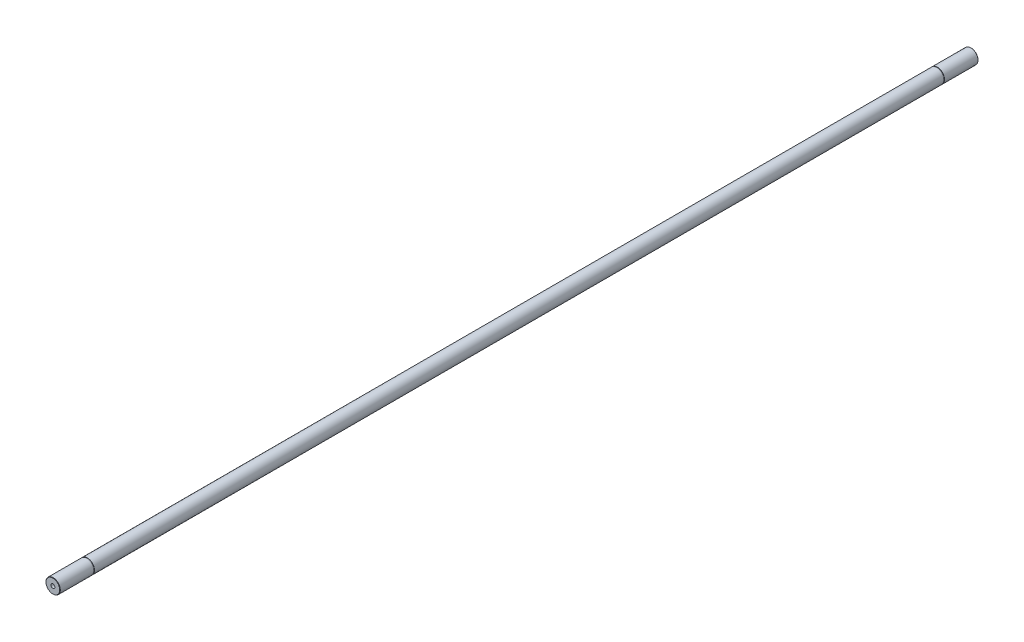
SolidWorks part; units mm, degrees
ref_plane "前视基准面" through (0, 0, 0) normal (0, 0, 1) x (1, 0, 0)
ref_plane "上视基准面" through (0, 0, 0) normal (0, 1, 0) x (1, 0, 0)
ref_plane "右视基准面" through (0, 0, 0) normal (1, 0, 0) x (0, 0, -1)
sketch "草图1" plane through (0, 0, 0) normal (0, 0, 1) x (1, 0, 0)
  circle A0 centre (0, 0) radius 12.5
  dimension "D1" = 25
extrude "凸台-拉伸1" add sketch "草图1" along normal blind 1600
chamfer "倒角1" distance 0.5 angle 45 2 edges at (12.5, 0, 0) (12.5, 0, 1600)
sketch "草图2" plane through (0, 0, 0) normal (0, 1, 0) x (1, 0, 0)
  line L0 (12.5, -1599.5) -> (12.5, -0.5) construction
  line L1 (12.5, -1539.9) -> (11.95, -1539.9)
  line L2 (12.5, -1539.9) -> (12.5, -1541.2)
  line L3 (12.5, -1541.2) -> (11.95, -1541.2)
  line L4 (11.95, -1539.9) -> (11.95, -1541.2)
  line L6 (0, -1599.5) -> (0, -1417.9402) construction
  line L7 (12.5, -1599.5) -> (-12.5, -1599.5) construction
  line L8 (12.5, -800) -> (406.5495, -800) construction
  line L9 (12.5, -1599.5) -> (12.5, -0.5) construction
  dimension "D1" = 1.3
  dimension "D2" = 0.55
  dimension "D3" = 739.9
revolve "切除-旋转1" cut sketch "草图2" angle 360 about L6
hole_wizard "M8 螺纹孔1" positions "草图4" profile "草图5" tap size "M8" standard "GB"
sketch "草图4" plane through (0, 0, 1600) normal (0, 0, 1) x (1, 0, 0)
  point P0 (0, 0)
sketch "草图5" plane through (0, 0, 1600) normal (1, 0, 0) x (0, -1, 0)
  line L0 (0, 0) -> (0, 21.7929)
  line L1 (0, 21.7929) -> (3.4, 19.75)
  line L2 (3.4, 19.75) -> (3.4, 0)
  line L5 (3.4, 0) -> (0, 0)
  line L10 (0, 21.7929) -> (-3.4, 19.75) construction
  line L11 (0, -6.35) -> (0, 107.95) construction
  dimension "螺纹孔钻头直径" = 6.8
  dimension "螺纹孔钻头深度" = 19.75
  dimension "导头角度" = 118
cosmetic thread "孔螺蚊线1" parameters "D1"=16, "D2"=8
ref_plane "基准面1" through (0, 0, 800) normal (0, 0, 1) x (1, 0, 0)
mirror "镜向1" about plane through (0, 0, 800) normal (0, 0, 1) of "M8 螺纹孔1", "切除-旋转1"
